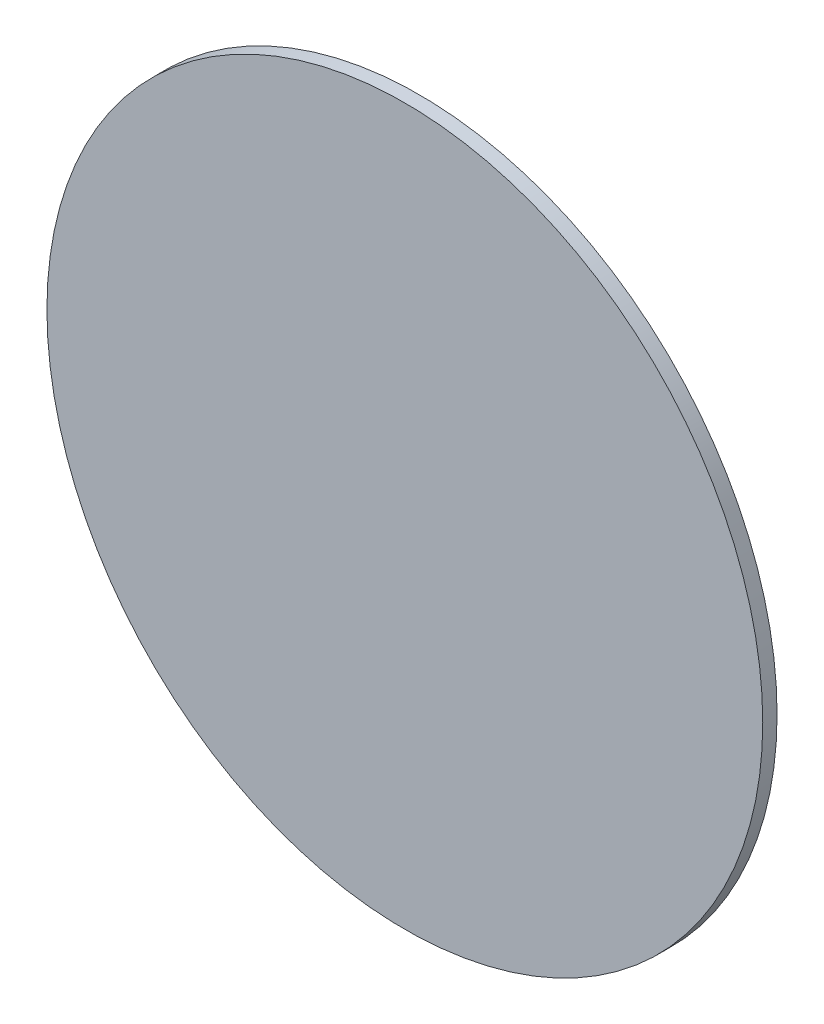
from build123d import *

# Parameters (mm, degrees)
SKETCH_1_R      = 25
EXTRUDE_1_DEPTH = 0.5


with BuildPart() as part:
    # 草图1 → 凸台-拉伸1 (new, symmetric)
    with BuildSketch(Plane.XY):
        Circle(SKETCH_1_R)
    extrude(amount=EXTRUDE_1_DEPTH, both=True)


solid = part.part
